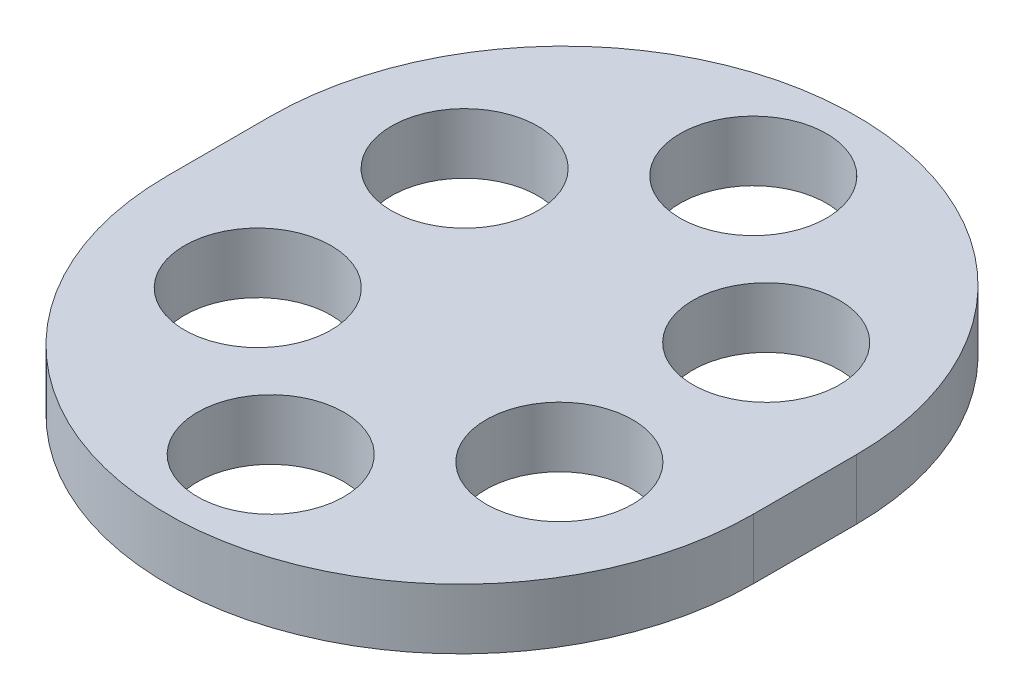
from build123d import *

# Parameters (mm, degrees)
SKETCH_1_R      = 8.5
EXTRUDE_1_DEPTH = 7


with BuildPart() as part:
    # 草图1 → 凸台-拉伸1 (new body)
    with BuildSketch(Plane(origin=(0, 0, 0), x_dir=(1, 0, 0), z_dir=(0, 1, 0))):
        with BuildLine():
            Line((34, -6), (34, 6))
            ThreePointArc((34, 6), (0, 40), (-34, 6))
            Line((-34, 6), (-34, -6))
            ThreePointArc((-34, -6), (0, -40), (34, -6))
        make_face()
        with Locations(Location((0, 28, 0), (0, 0, 270))):
            Circle(SKETCH_1_R, mode=Mode.SUBTRACT)
        with Locations(Location((-17.5, 12, 0), (0, 0, 270))):
            Circle(SKETCH_1_R, mode=Mode.SUBTRACT)
        with Locations(Location((17.5, 12, 0), (0, 0, 90))):
            Circle(SKETCH_1_R, mode=Mode.SUBTRACT)
        with Locations(Location((17.5, -12, 0), (0, 0, 270))):
            Circle(SKETCH_1_R, mode=Mode.SUBTRACT)
        with Locations(Location((-17.5, -12, 0), (0, 0, 90))):
            Circle(SKETCH_1_R, mode=Mode.SUBTRACT)
        with Locations(Location((0, -28, 0), (0, 0, 90))):
            Circle(SKETCH_1_R, mode=Mode.SUBTRACT)
    extrude(amount=EXTRUDE_1_DEPTH)


solid = part.part
